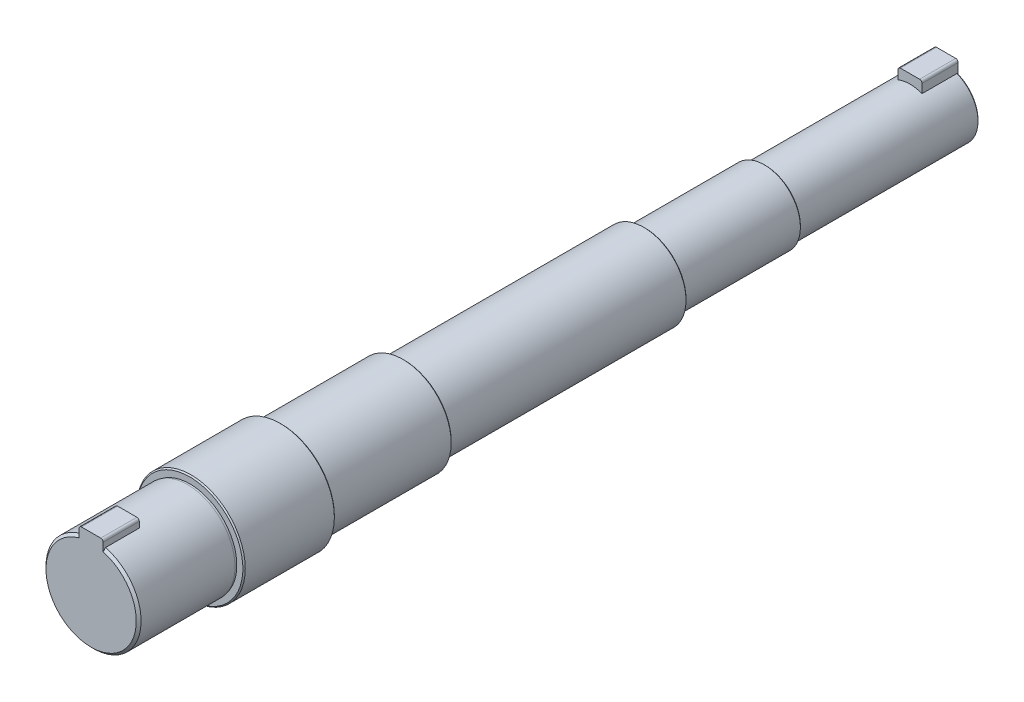
from build123d import *

# Parameters (mm, degrees)
SKETCH1_R            = 3.95
BOSS_EXTRUDE1_DEPTH  = 8
SKETCH2_W            = 2
SKETCH2_H            = 1.5
BOSS_EXTRUDE2_DEPTH  = 3
FILLET1_R            = 0.2
SKETCH3_R            = 3.9
BOSS_EXTRUDE3_DEPTH  = 0.2
SKETCH4_R            = 4.5
BOSS_EXTRUDE4_DEPTH  = 7.6
SKETCH6_R            = 3.9
BOSS_EXTRUDE5_DEPTH  = 0.2
CHAMFER2_SIZE        = 0.2
SKETCH7_R            = 4
BOSS_EXTRUDE8_DEPTH  = 10
SKETCH9_R            = 3.5
BOSS_EXTRUDE9_DEPTH  = 20
SKETCH10_R           = 3
BOSS_EXTRUDE10_DEPTH = 10
SKETCH13_R           = 2.75
BOSS_EXTRUDE11_DEPTH = 15
BOSS_EXTRUDE13_DEPTH = 3
FILLET2_R            = 0.2
CHAMFER5_SIZE        = 0.1


with BuildPart() as part:
    # Sketch1 → Boss-Extrude1 (new body)
    with BuildSketch(Plane.XY):
        Circle(SKETCH1_R)
    extrude(amount=BOSS_EXTRUDE1_DEPTH)

    # Sketch2 → Boss-Extrude2 (add)
    with BuildSketch(Plane(origin=(0, 0, 5), x_dir=(-1, 0, 0), z_dir=(0, 0, -1))):
        with Locations((0, 3.75)):
            Rectangle(SKETCH2_W, SKETCH2_H)
    extrude(amount=-BOSS_EXTRUDE2_DEPTH)

    # Fillet1
    fillet1_edges = [part.edges().sort_by_distance(p)[0] for p in [
        (-1, 4.5, 6.5),
        (1, 4.5, 6.5),
    ]]
    fillet(fillet1_edges, radius=FILLET1_R)

    # Sketch3 → Boss-Extrude3 (add)
    with BuildSketch(Plane(origin=(0, 0, 0), x_dir=(-1, 0, 0), z_dir=(0, 0, -1))):
        Circle(SKETCH3_R)
    extrude(amount=BOSS_EXTRUDE3_DEPTH)

    # Sketch4 → Boss-Extrude4 (add)
    with BuildSketch(Plane(origin=(0, 0, -0.2), x_dir=(-1, 0, 0), z_dir=(0, 0, -1))):
        with Locations(Location((0, 0, 0), (0, 0, 180))):
            Circle(SKETCH4_R)
    extrude(amount=BOSS_EXTRUDE4_DEPTH)

    # Sketch6 → Boss-Extrude5 (add)
    with BuildSketch(Plane(origin=(0, 0, -7.8), x_dir=(-1, 0, 0), z_dir=(0, 0, -1))):
        Circle(SKETCH6_R)
    extrude(amount=BOSS_EXTRUDE5_DEPTH)

    # Chamfer2
    chamfer2_edges = [part.edges().sort_by_distance(p)[0] for p in [
        (-2.413762623, -3.126699538, 8),
    ]]
    chamfer(chamfer2_edges, length=CHAMFER2_SIZE)

    # Sketch7 → Boss-Extrude8 (add)
    with BuildSketch(Plane(origin=(0, 0, -8), x_dir=(-1, 0, 0), z_dir=(0, 0, -1))):
        Circle(SKETCH7_R)
    extrude(amount=BOSS_EXTRUDE8_DEPTH)

    # Sketch9 → Boss-Extrude9 (add)
    with BuildSketch(Plane(origin=(0, 0, -18), x_dir=(-1, 0, 0), z_dir=(0, 0, -1))):
        Circle(SKETCH9_R)
    extrude(amount=BOSS_EXTRUDE9_DEPTH)

    # Sketch10 → Boss-Extrude10 (add)
    with BuildSketch(Plane(origin=(0, 0, -38), x_dir=(-1, 0, 0), z_dir=(0, 0, -1))):
        Circle(SKETCH10_R)
    extrude(amount=BOSS_EXTRUDE10_DEPTH)

    # Sketch13 → Boss-Extrude11 (add)
    with BuildSketch(Plane(origin=(0, 0, -48), x_dir=(-1, 0, 0), z_dir=(0, 0, -1))):
        Circle(SKETCH13_R)
    extrude(amount=BOSS_EXTRUDE11_DEPTH)

    # Sketch14 → Boss-Extrude13 (add)
    with BuildSketch(Plane(origin=(0, 0, -60), x_dir=(-1, 0, 0), z_dir=(0, 0, -1))):
        with BuildLine():
            Line((-1, 3.5), (1, 3.5))
            Line((1, 3.5), (1, 2.561737691))
            ThreePointArc((1, 2.561737691), (0, 2.75), (-1, 2.561737691))
            Line((-1, 2.561737691), (-1, 3.5))
        make_face()
    extrude(amount=BOSS_EXTRUDE13_DEPTH)

    # Fillet2
    fillet2_edges = [part.edges().sort_by_distance(p)[0] for p in [
        (-1, 3.5, -61.5),
        (1, 3.5, -61.5),
    ]]
    fillet(fillet2_edges, radius=FILLET2_R)

    # Chamfer5
    chamfer5_edges = [part.edges().sort_by_distance(p)[0] for p in [
        (-4.5, 0, -0.2),
        (-4.5, 0, -7.8),
        (4, 0, -18),
        (3.5, 0, -38),
        (3, 0, -48),
        (1.551209206, -2.270737766, -63),
    ]]
    chamfer(chamfer5_edges, length=CHAMFER5_SIZE)


solid = part.part
